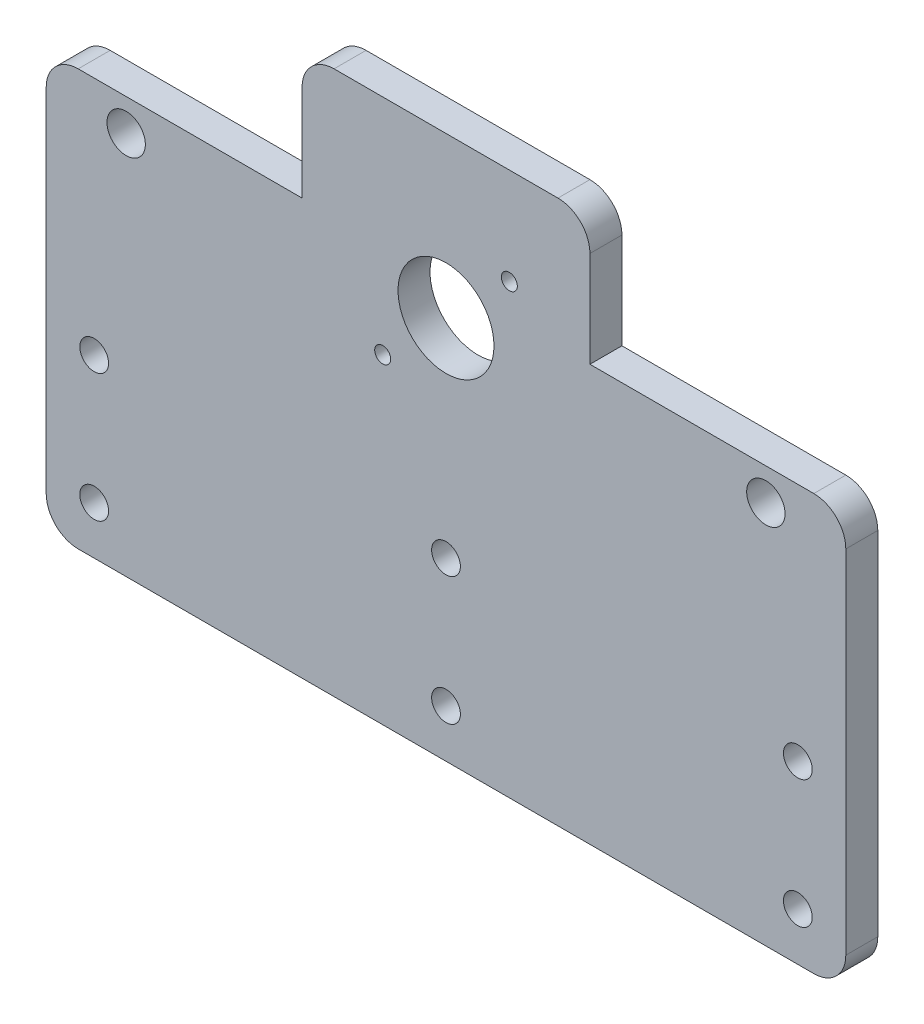
SolidWorks part; units mm, degrees
ref_plane "前视基准面" through (0, 0, 0) normal (0, 0, 1) x (1, 0, 0)
ref_plane "上视基准面" through (0, 0, 0) normal (0, 1, 0) x (1, 0, 0)
ref_plane "右视基准面" through (0, 0, 0) normal (1, 0, 0) x (0, 0, -1)
sketch "草图1" plane through (0, 0, 0) normal (0, 0, 1) x (1, 0, 0)
  line L1 (-125, 85) -> (125, 85)
  line L2 (-125, 85) -> (-125, -85)
  line L3 (-125, -85) -> (125, -85)
  line L4 (125, 85) -> (125, -85)
  line L5 (-125, 85) -> (125, -85) construction
  line L6 (-125, -85) -> (125, 85) construction
  point P0 (0, 0)
  dimension "D1" = 250
  dimension "D2" = 170
extrude "凸台-拉伸1" add sketch "草图1" along normal mid plane 10
sketch "草图2" plane through (0, 0, 5) normal (0, 0, 1) x (1, 0, 0)
  line L0 (125, 85) -> (-125, 85) construction
  line L1 (45, 85) -> (125, 85)
  line L2 (45, 85) -> (45, 45)
  line L3 (45, 45) -> (125, 45)
  line L4 (125, 85) -> (125, 45)
  line L5 (125, -85) -> (125, 85) construction
  dimension "D1" = 80
  dimension "D2" = 40
extrude "切除-拉伸1" cut sketch "草图2" against normal blind 10
mirror "镜向1" about plane through (0, 0, 0) normal (1, 0, 0) of "切除-拉伸1"
hole_wizard "Ø9.0 (9) 直径孔1" positions "草图4" profile "草图3" hole size "Ø9.0" standard "GB" end condition up to next
sketch "草图4" plane through (0, 0, 5) normal (0, 0, 1) x (1, 0, 0)
  line L0 (-125, -85) -> (125, -85) construction
  line L1 (-125, 45) -> (-125, -85) construction
  point P0 (-110, -30)
  point P2 (-110, -70)
  dimension "D1" = 15
  dimension "D2" = 40
  dimension "D3" = 15
sketch "草图3" plane through (-110, -30, 5) normal (1, 0, 0) x (0, -1, 0)
  line L0 (0, 0) -> (0, 10)
  line L1 (0, 10) -> (4.5, 10)
  line L2 (4.5, 10) -> (4.5, 0)
  line L5 (4.5, 0) -> (0, 0)
  line L11 (0, -6.35) -> (0, 107.95) construction
  dimension "通孔孔直径" = 9
  dimension "通孔孔深度" = 10
pattern_linear "阵列(线性)1" count 3 spacing 110 along (1, 0, 0) of "Ø9.0 (9) 直径孔1"
hole_wizard "Ø12.0 (12) 直径孔1" positions "草图6" profile "草图5" hole size "Ø12.0" standard "GB" end condition up to next
sketch "草图6" plane through (0, 0, 5) normal (0, 0, 1) x (1, 0, 0)
  line L0 (-125, -85) -> (125, -85) construction
  point P0 (-100, 35)
  point P2 (100, 35)
  dimension "D1" = 200
  dimension "D2" = 100
  dimension "D3" = 120
sketch "草图5" plane through (-100, 35, 5) normal (1, 0, 0) x (0, -1, 0)
  line L0 (0, 0) -> (0, 10)
  line L1 (0, 10) -> (6, 10)
  line L2 (6, 10) -> (6, 0)
  line L5 (6, 0) -> (0, 0)
  line L11 (0, -6.35) -> (0, 107.95) construction
  dimension "通孔孔直径" = 12
  dimension "通孔孔深度" = 10
sketch "草图7" plane through (0, 0, 5) normal (0, 0, 1) x (1, 0, 0)
  line L0 (-125, -85) -> (125, -85) construction
  circle A0 centre (0, 35) radius 15
  dimension "D1" = 30
  dimension "D2" = 120
extrude "切除-拉伸2" cut sketch "草图7" against normal blind 10
hole_wizard "M6 螺纹孔1" positions "草图9" profile "草图8" tap size "M6" standard "ISO" end condition up to next
sketch "草图9" plane through (0, 0, 5) normal (0, 0, 1) x (1, 0, 0)
  circle A1 centre (0, 35) radius 15 construction
  point P0 (-19.8, 15.2)
  point P2 (19.8, 54.8)
  dimension "D1" = 39.6
  dimension "D2" = 39.6
  dimension "D3" = 19.8
  dimension "D4" = 19.8
sketch "草图8" plane through (-19.8, 15.2, 5) normal (1, 0, 0) x (0, -1, 0)
  line L0 (0, 0) -> (0, 10)
  line L1 (0, 10) -> (2.5, 10)
  line L2 (2.5, 10) -> (2.5, 0)
  line L5 (2.5, 0) -> (0, 0)
  line L11 (0, -6.35) -> (0, 107.95) construction
  dimension "通孔螺纹孔钻头直径" = 5
  dimension "通孔螺纹孔钻头深度" = 10
cosmetic thread "孔螺蚊线1" parameters "D2"=6
cosmetic thread "孔螺蚊线2" parameters "D2"=6
fillet "圆角1" radius 10 6 edges at (125, -85, 0) (125, 45, 0) (45, 85, 0) (-45, 85, 0) (-125, -85, 0) (-125, 45, 0)
